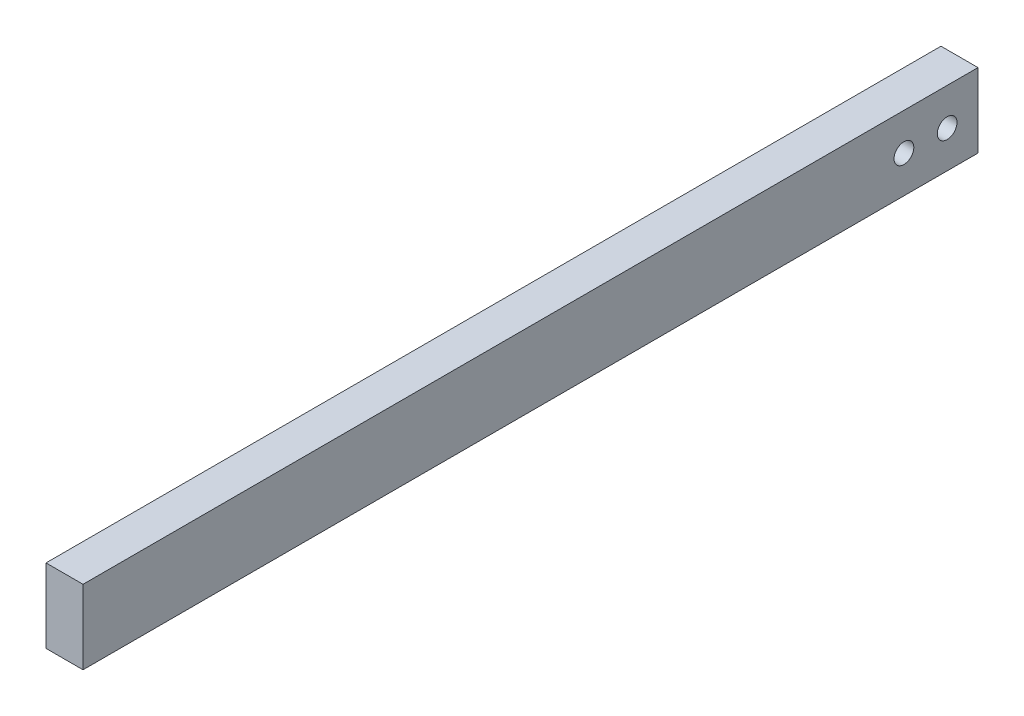
from build123d import *

# Parameters (mm, degrees)
SKETCH_1_W          = 30
SKETCH_1_H          = 60
EXTRUDE_1_DEPTH     = 642
SKETCH_2_W          = 30
SKETCH_2_H          = 60
EXTRUDE_2_DEPTH     = 83
SKETCH_3_R          = 8
CUT_EXTRUDE_1_DEPTH = 644.400341933


with BuildPart() as part:
    # 草图1 → 凸台-拉伸1 (new body)
    with BuildSketch(Plane.XY):
        Rectangle(SKETCH_1_W, SKETCH_1_H)
    extrude(amount=EXTRUDE_1_DEPTH)

    # 草图2 → 凸台-拉伸2 (add)
    with BuildSketch(Plane(origin=(0, 0, 0), x_dir=(-1, 0, 0), z_dir=(0, 0, -1))):
        Rectangle(SKETCH_2_W, SKETCH_2_H)
    extrude(amount=EXTRUDE_2_DEPTH)

    # 草图3 → 切除-拉伸1 (cut, through all)
    with BuildSketch(Plane.ZY.offset(15)):
        with Locations((-58, 0)):
            Circle(SKETCH_3_R)
        with Locations((-23, 0)):
            Circle(SKETCH_3_R)
    extrude(amount=-CUT_EXTRUDE_1_DEPTH, mode=Mode.SUBTRACT)


solid = part.part
